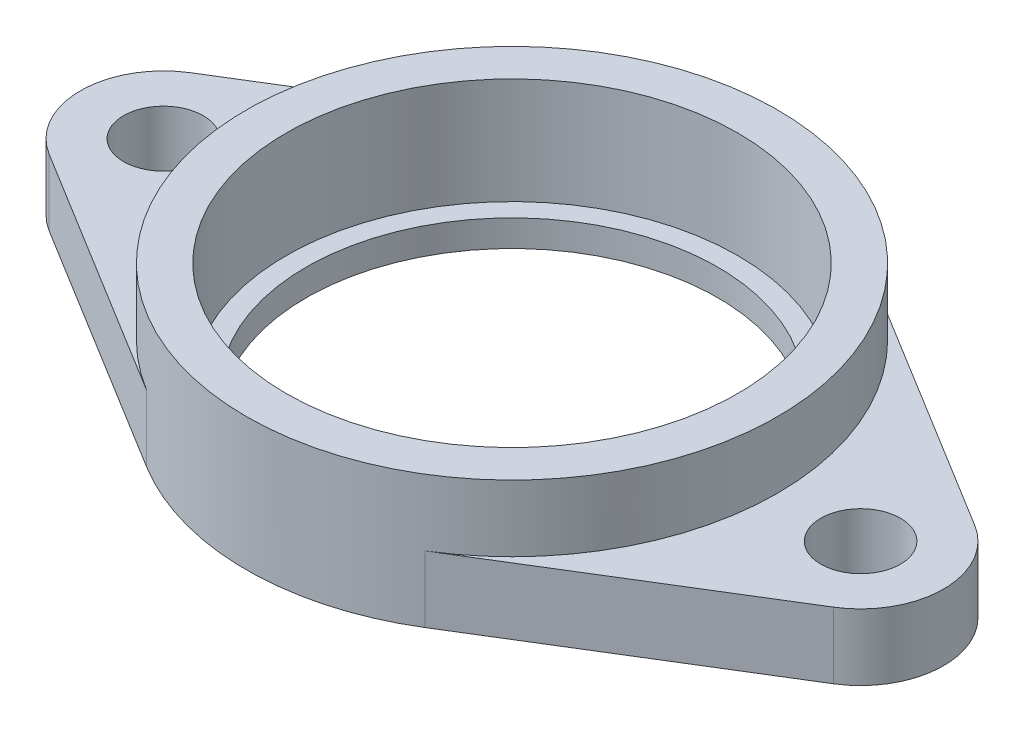
from build123d import *
from build123d.topology import SkipClean

# Parameters (mm, degrees)
SKETCH_1_R          = 6
EXTRUDE_1_DEPTH     = 10
SKETCH_2_R          = 40
EXTRUDE_2_DEPTH     = 10
SKETCH_3_R          = 34
CUT_EXTRUDE_1_DEPTH = 16
SKETCH_4_R          = 31
CUT_EXTRUDE_2_DEPTH = 16


with BuildPart() as part:
    # 草图1 → 凸台-拉伸1 (new body)
    with BuildSketch(Plane(origin=(0, 0, 0), x_dir=(1, 0, 0), z_dir=(0, 1, 0))):
        with BuildLine():
            Line((-59.047619048, 10.64794275), (-20.952380952, 34.0734168))
            ThreePointArc((-20.952380952, 34.0734168), (0, 40), (20.952380952, 34.0734168))
            Line((20.952380952, 34.0734168), (59.047619048, 10.64794275))
            ThreePointArc((59.047619048, 10.64794275), (65, 0), (59.047619048, -10.64794275))
            Line((59.047619048, -10.64794275), (20.952380952, -34.0734168))
            ThreePointArc((20.952380952, -34.0734168), (0, -40), (-20.952380952, -34.0734168))
            Line((-20.952380952, -34.0734168), (-59.047619048, -10.64794275))
            ThreePointArc((-59.047619048, -10.64794275), (-65, 0), (-59.047619048, 10.64794275))
        make_face()
        with Locations(Location((52.5, 0, 0), (0, 0, 270))):
            Circle(SKETCH_1_R, mode=Mode.SUBTRACT)
        with Locations(Location((-52.5, 0, 0), (0, 0, 270))):
            Circle(SKETCH_1_R, mode=Mode.SUBTRACT)
    extrude(amount=EXTRUDE_1_DEPTH)

    # 草图2 → 凸台-拉伸2 (add)
    with SkipClean():  # the faces are left unmerged after this step: merging them gives an invalid solid
        with BuildSketch(Plane(origin=(0, 10, 0), x_dir=(1, 0, 0), z_dir=(0, 1, 0))):
            with Locations(Location((0, 0, 0), (0, 0, 121.588135505))):
                Circle(SKETCH_2_R)
        extrude(amount=EXTRUDE_2_DEPTH)

    # 草图3 → 切除-拉伸1 (cut)
    with SkipClean():  # the faces are left unmerged after this step: merging them gives an invalid solid
        with BuildSketch(Plane(origin=(0, 20, 0), x_dir=(1, 0, 0), z_dir=(0, 1, 0))):
            with Locations(Location((0, 0, 0), (0, 0, 270))):
                Circle(SKETCH_3_R)
        extrude(amount=-CUT_EXTRUDE_1_DEPTH, mode=Mode.SUBTRACT)

    # 草图4 → 切除-拉伸2 (cut)
    with SkipClean():  # the faces are left unmerged after this step: merging them gives an invalid solid
        with BuildSketch(Plane(origin=(0, 4, 0), x_dir=(1, 0, 0), z_dir=(0, 1, 0))):
            with Locations(Location((0, 0, 0), (0, 0, 270))):
                Circle(SKETCH_4_R)
        extrude(amount=-CUT_EXTRUDE_2_DEPTH, mode=Mode.SUBTRACT)


solid = part.part
